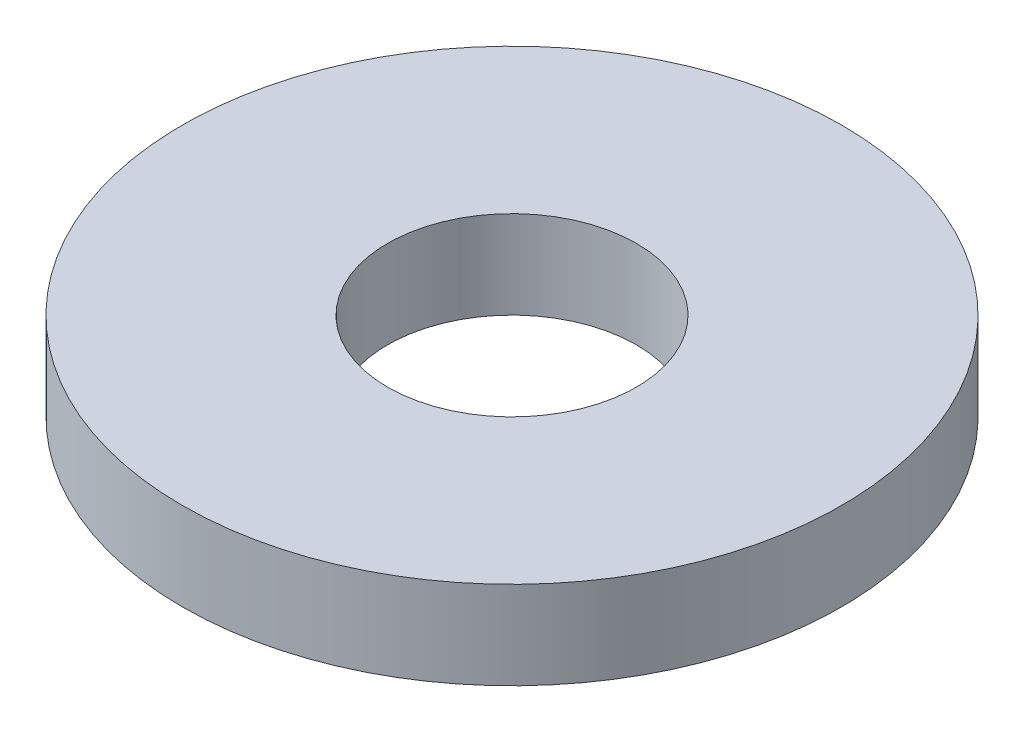
SolidWorks part; units mm, degrees
ref_plane "Front Plane" through (0, 0, 0) normal (0, 0, 1) x (1, 0, 0)
ref_plane "Top Plane" through (0, 0, 0) normal (0, 1, 0) x (1, 0, 0)
ref_plane "Right Plane" through (0, 0, 0) normal (1, 0, 0) x (0, 0, -1)
sketch "Sketch1" plane through (0, 0, 0) normal (0, 1, 0) x (1, 0, 0)
  circle A0 centre (0, 0) radius 22.5
  circle A1 centre (0, 0) radius 8.5
extrude "Boss-Extrude1" add sketch "Sketch1" along normal blind 6
